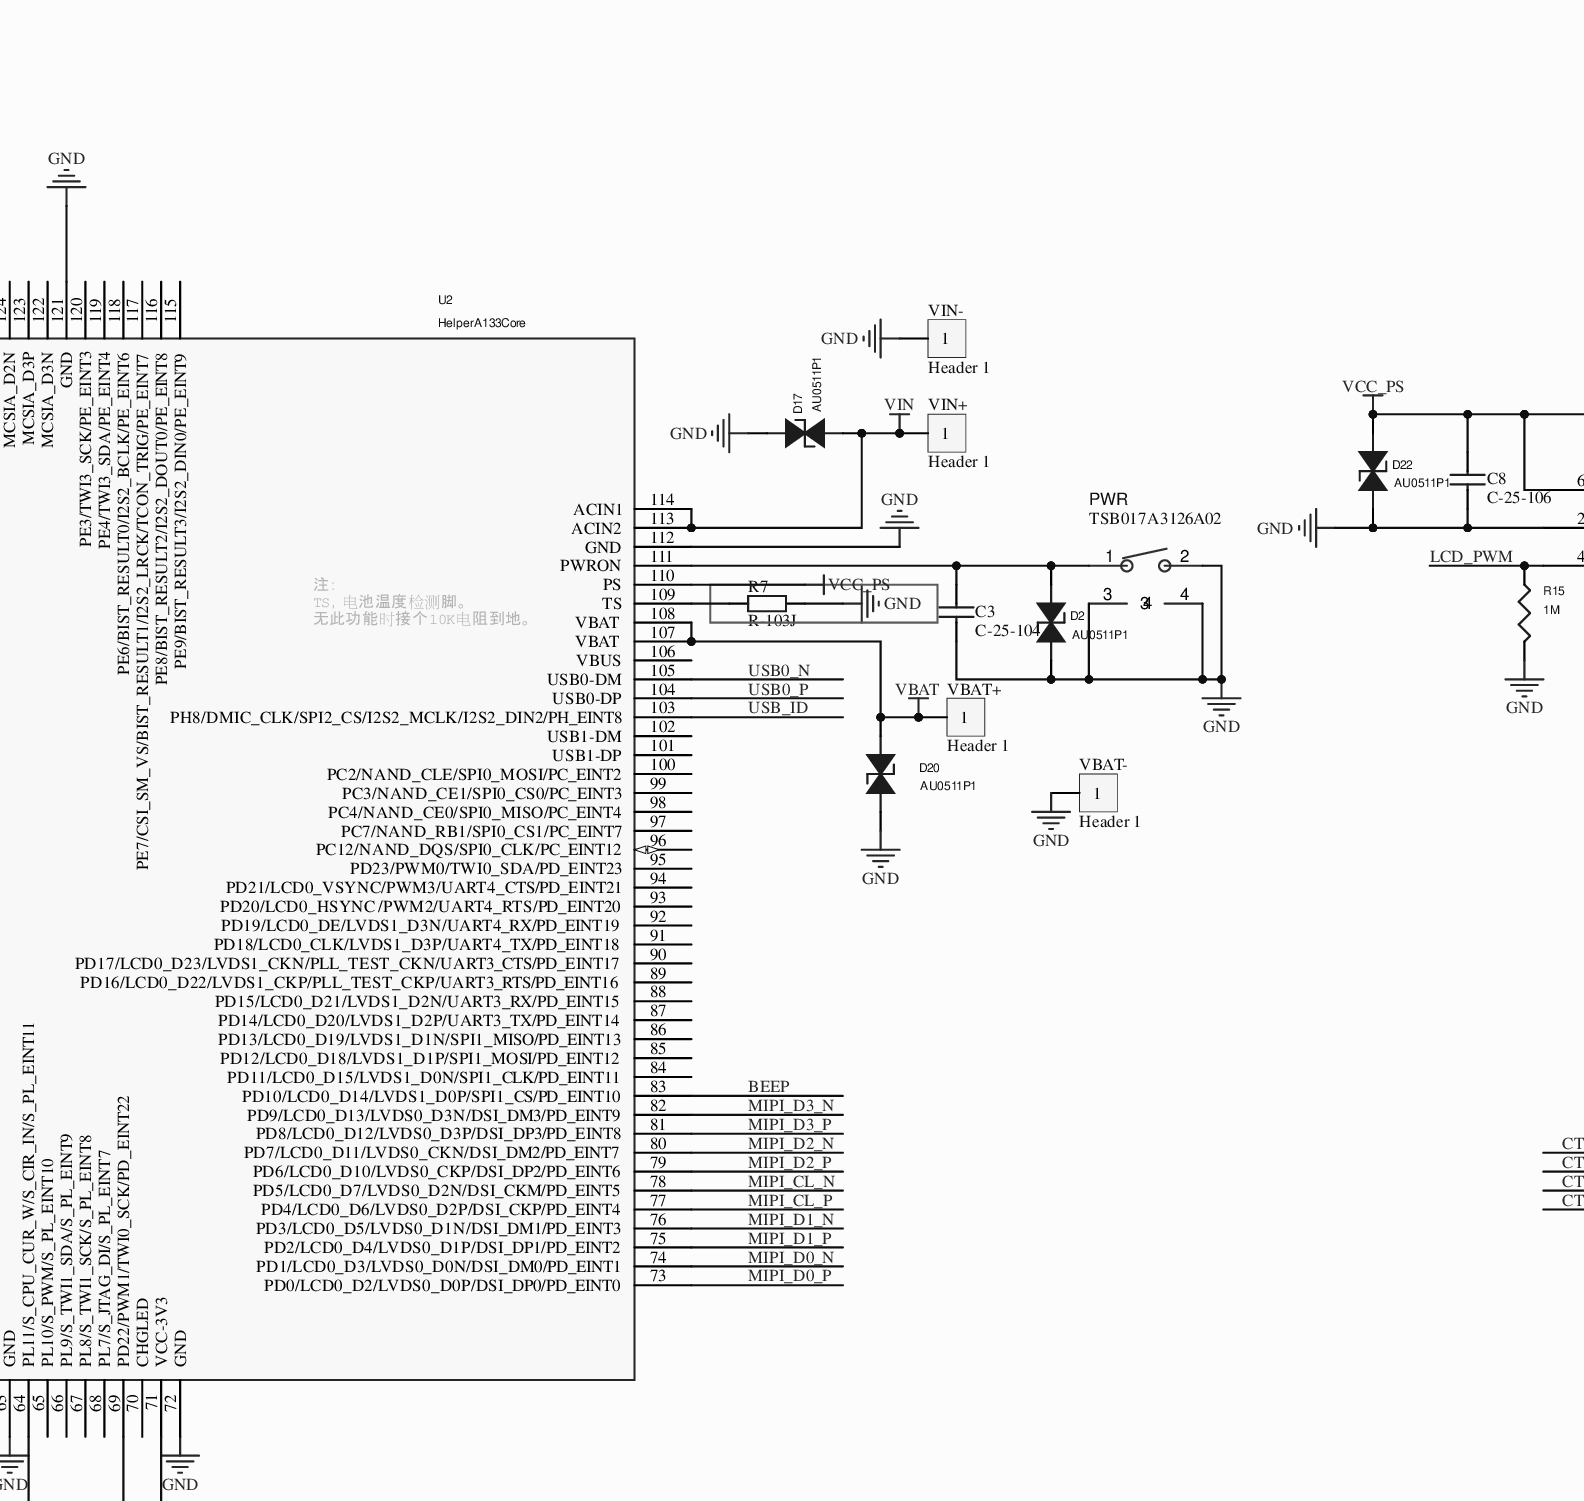
[diagram p0: MISC105407.SchDoc, centre column 3 of 4]
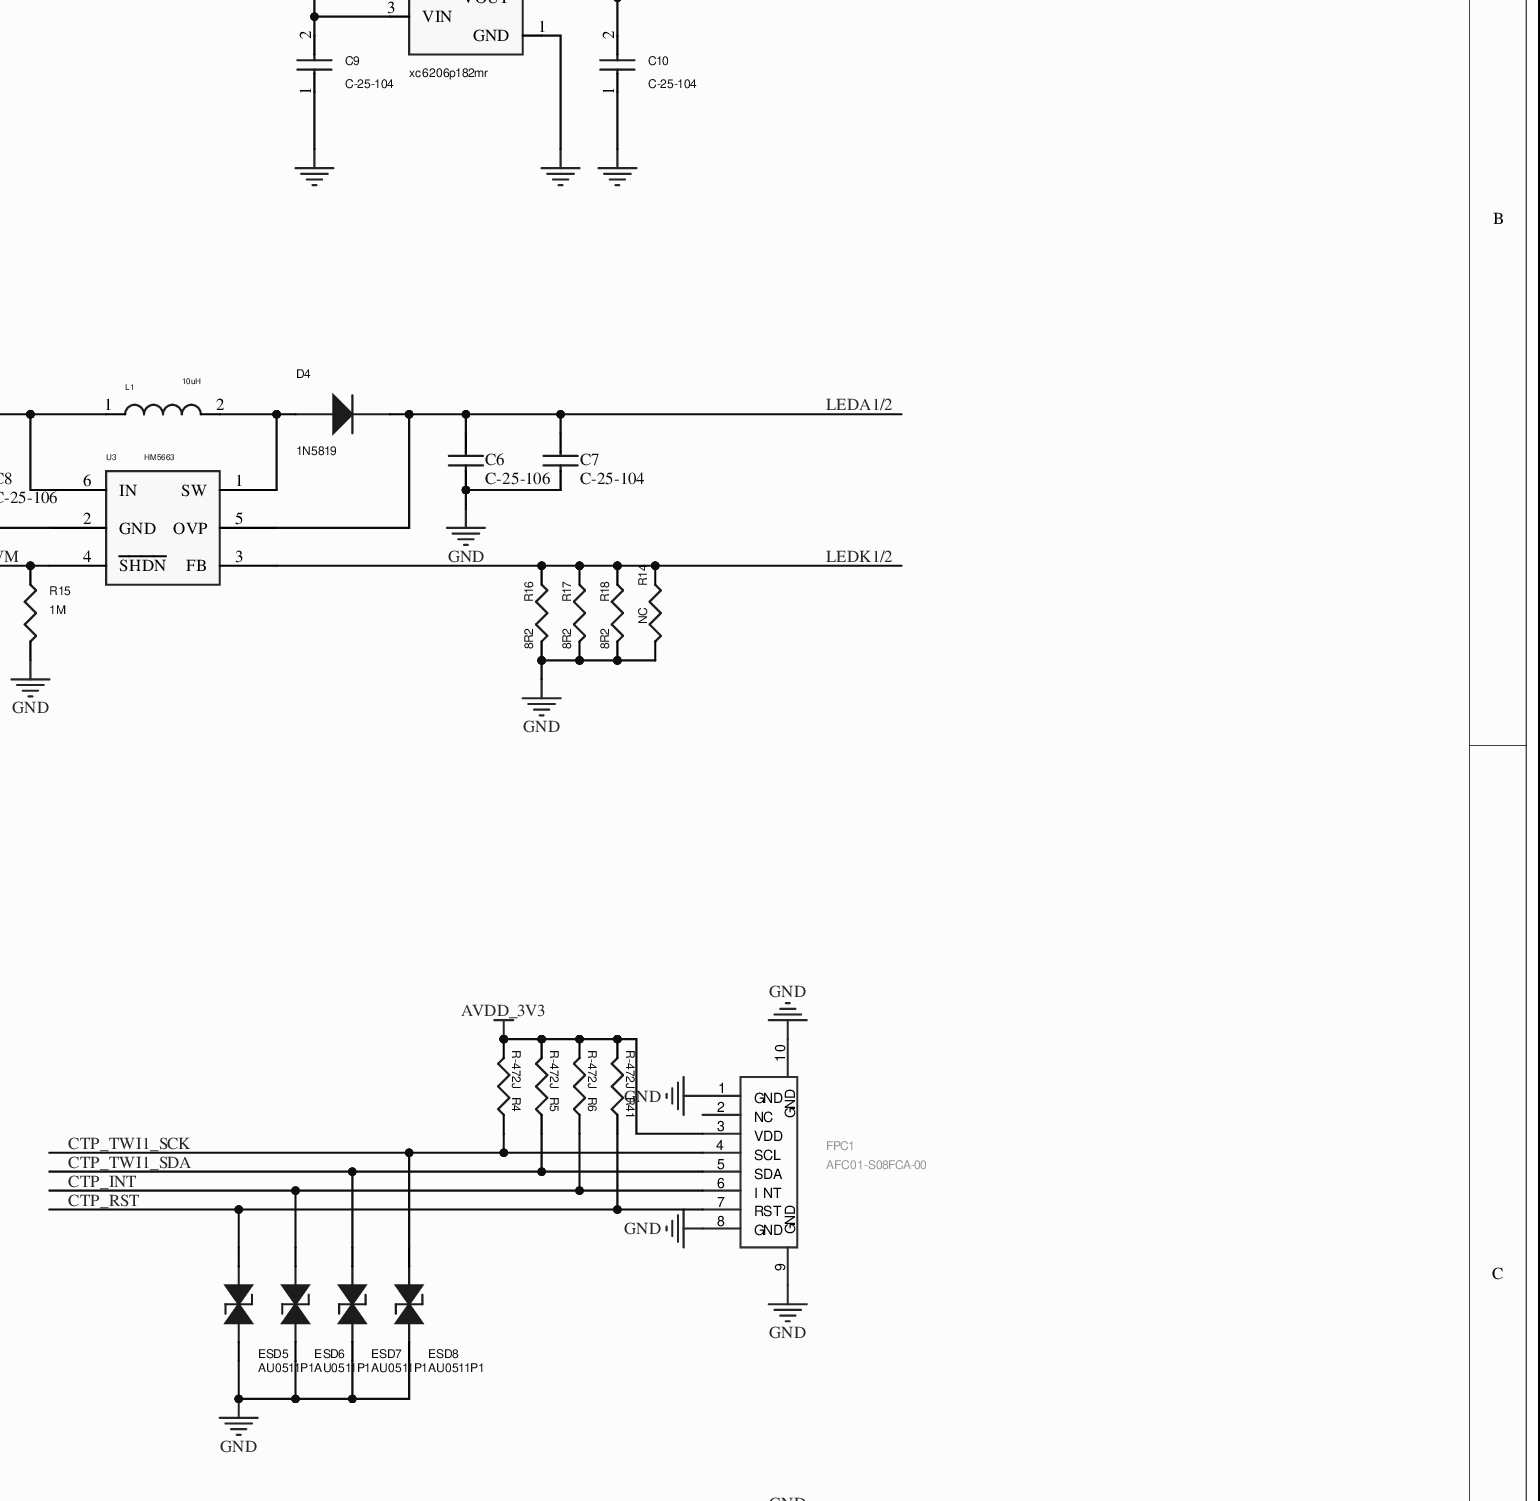
[diagram p1: MISC105407.SchDoc, centre column 4 of 4]
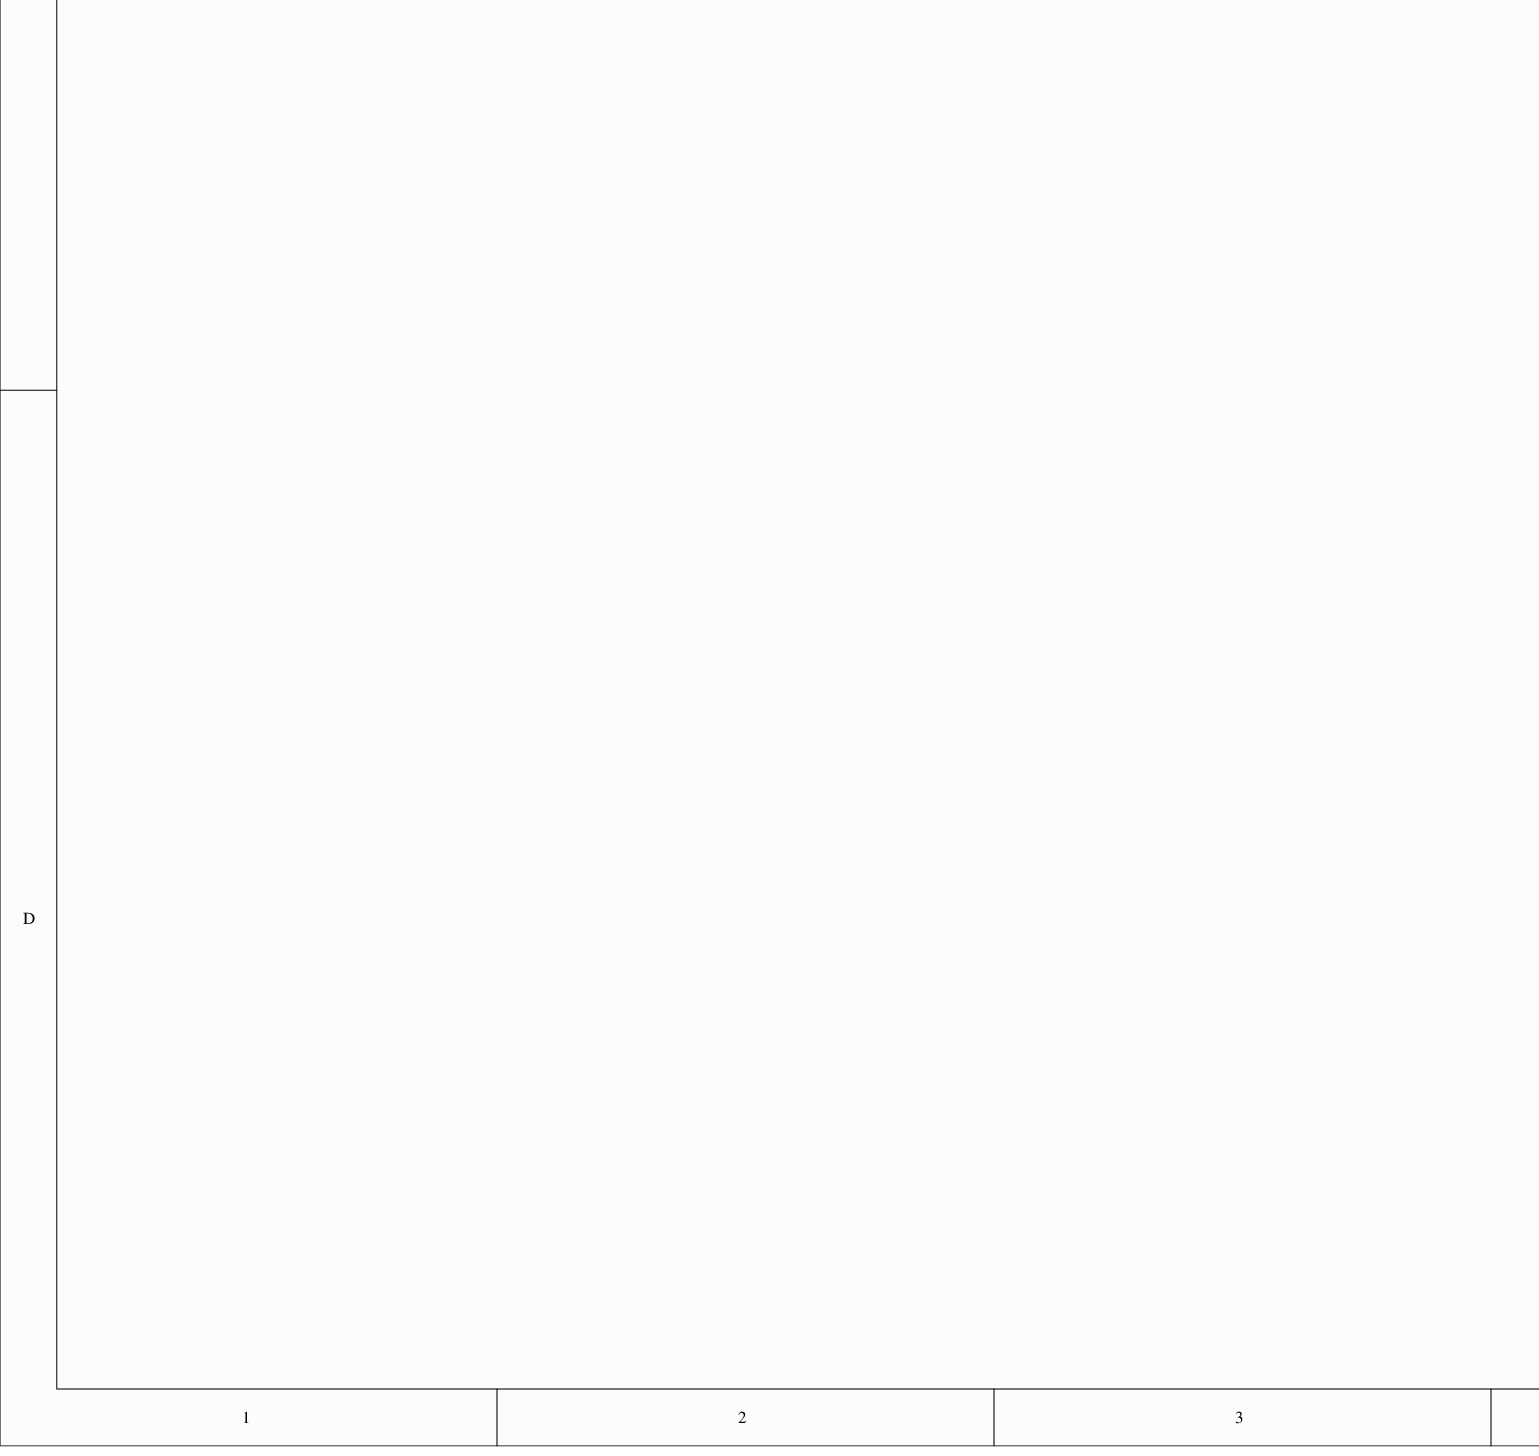
[diagram p2: MISC105407.SchDoc, bottom column 1 of 4]
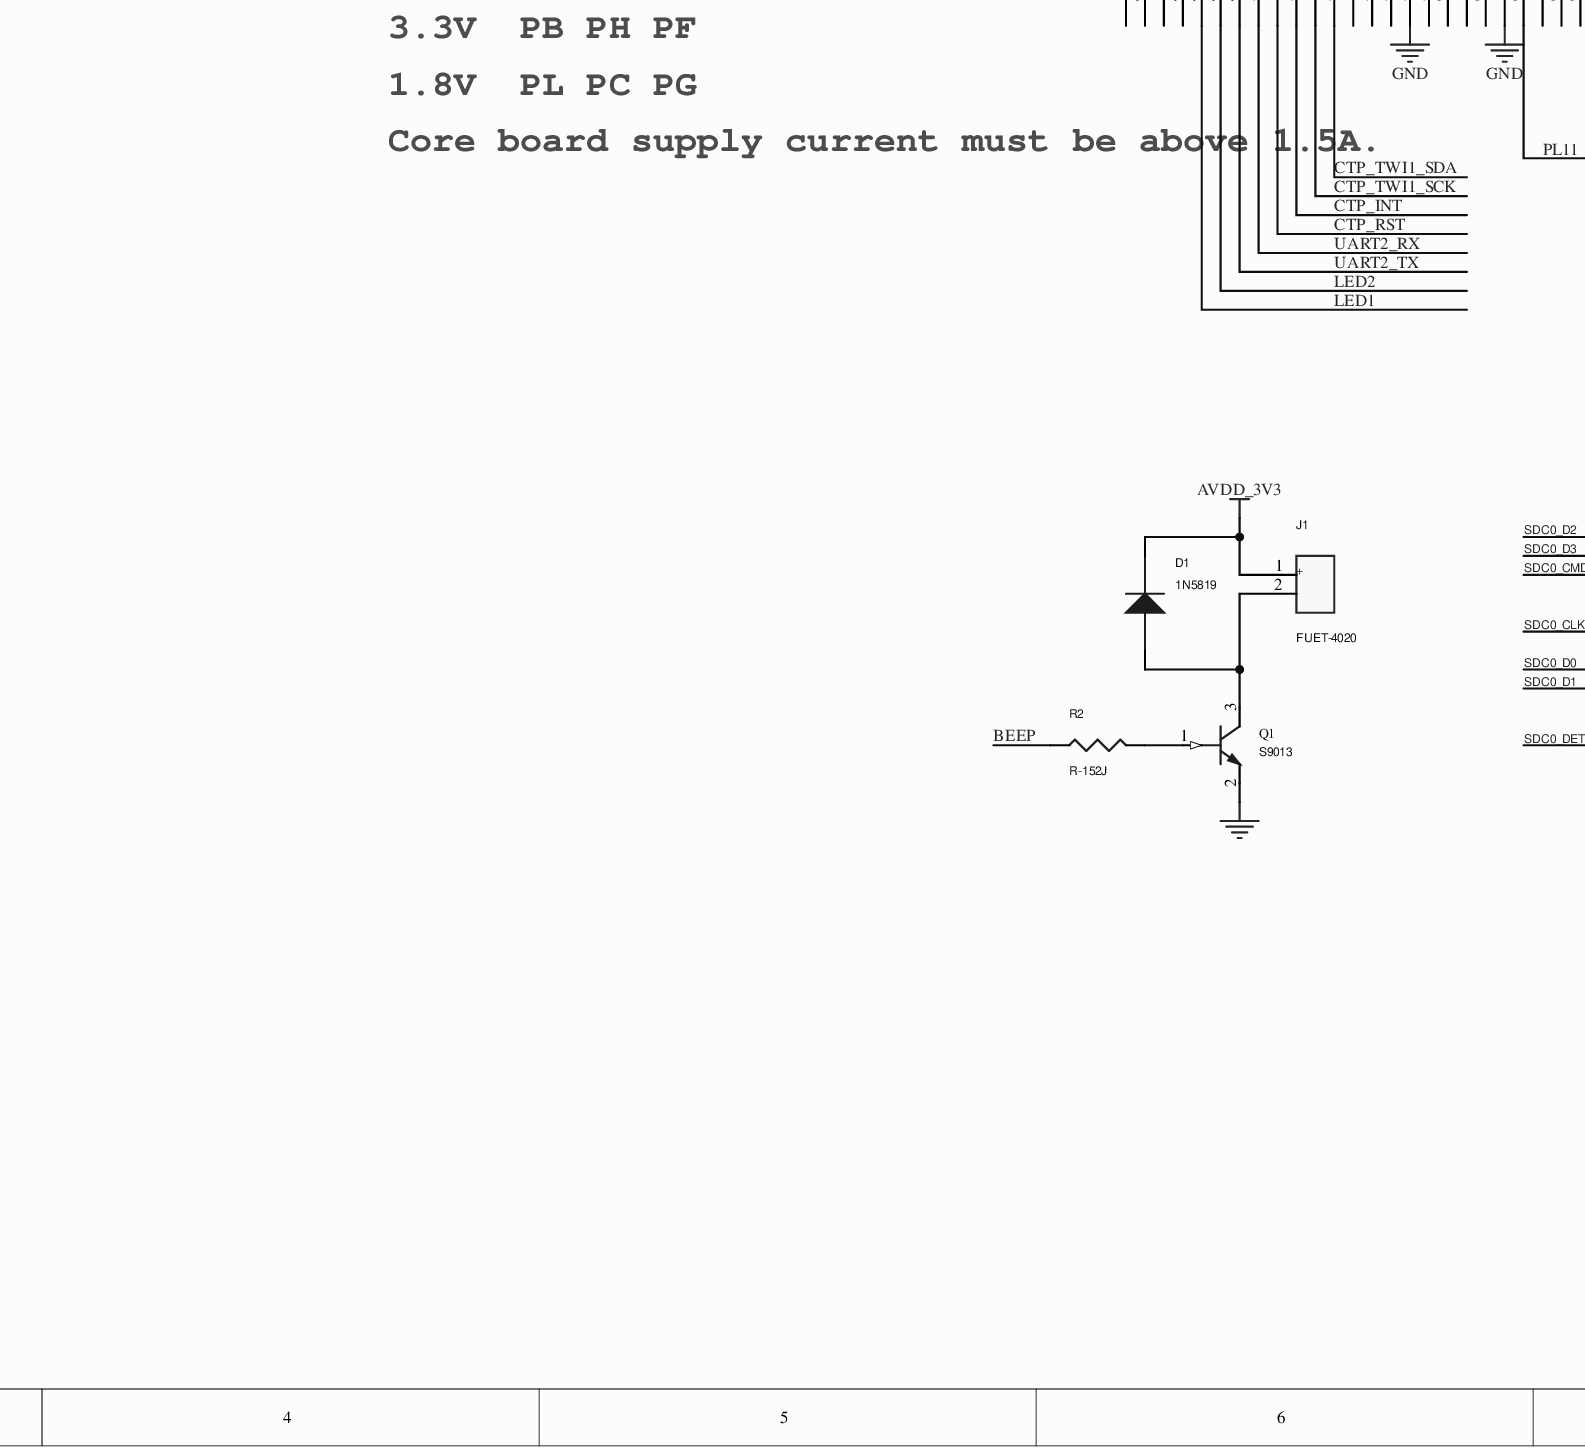
[diagram p3: MISC105407.SchDoc, bottom column 2 of 4]
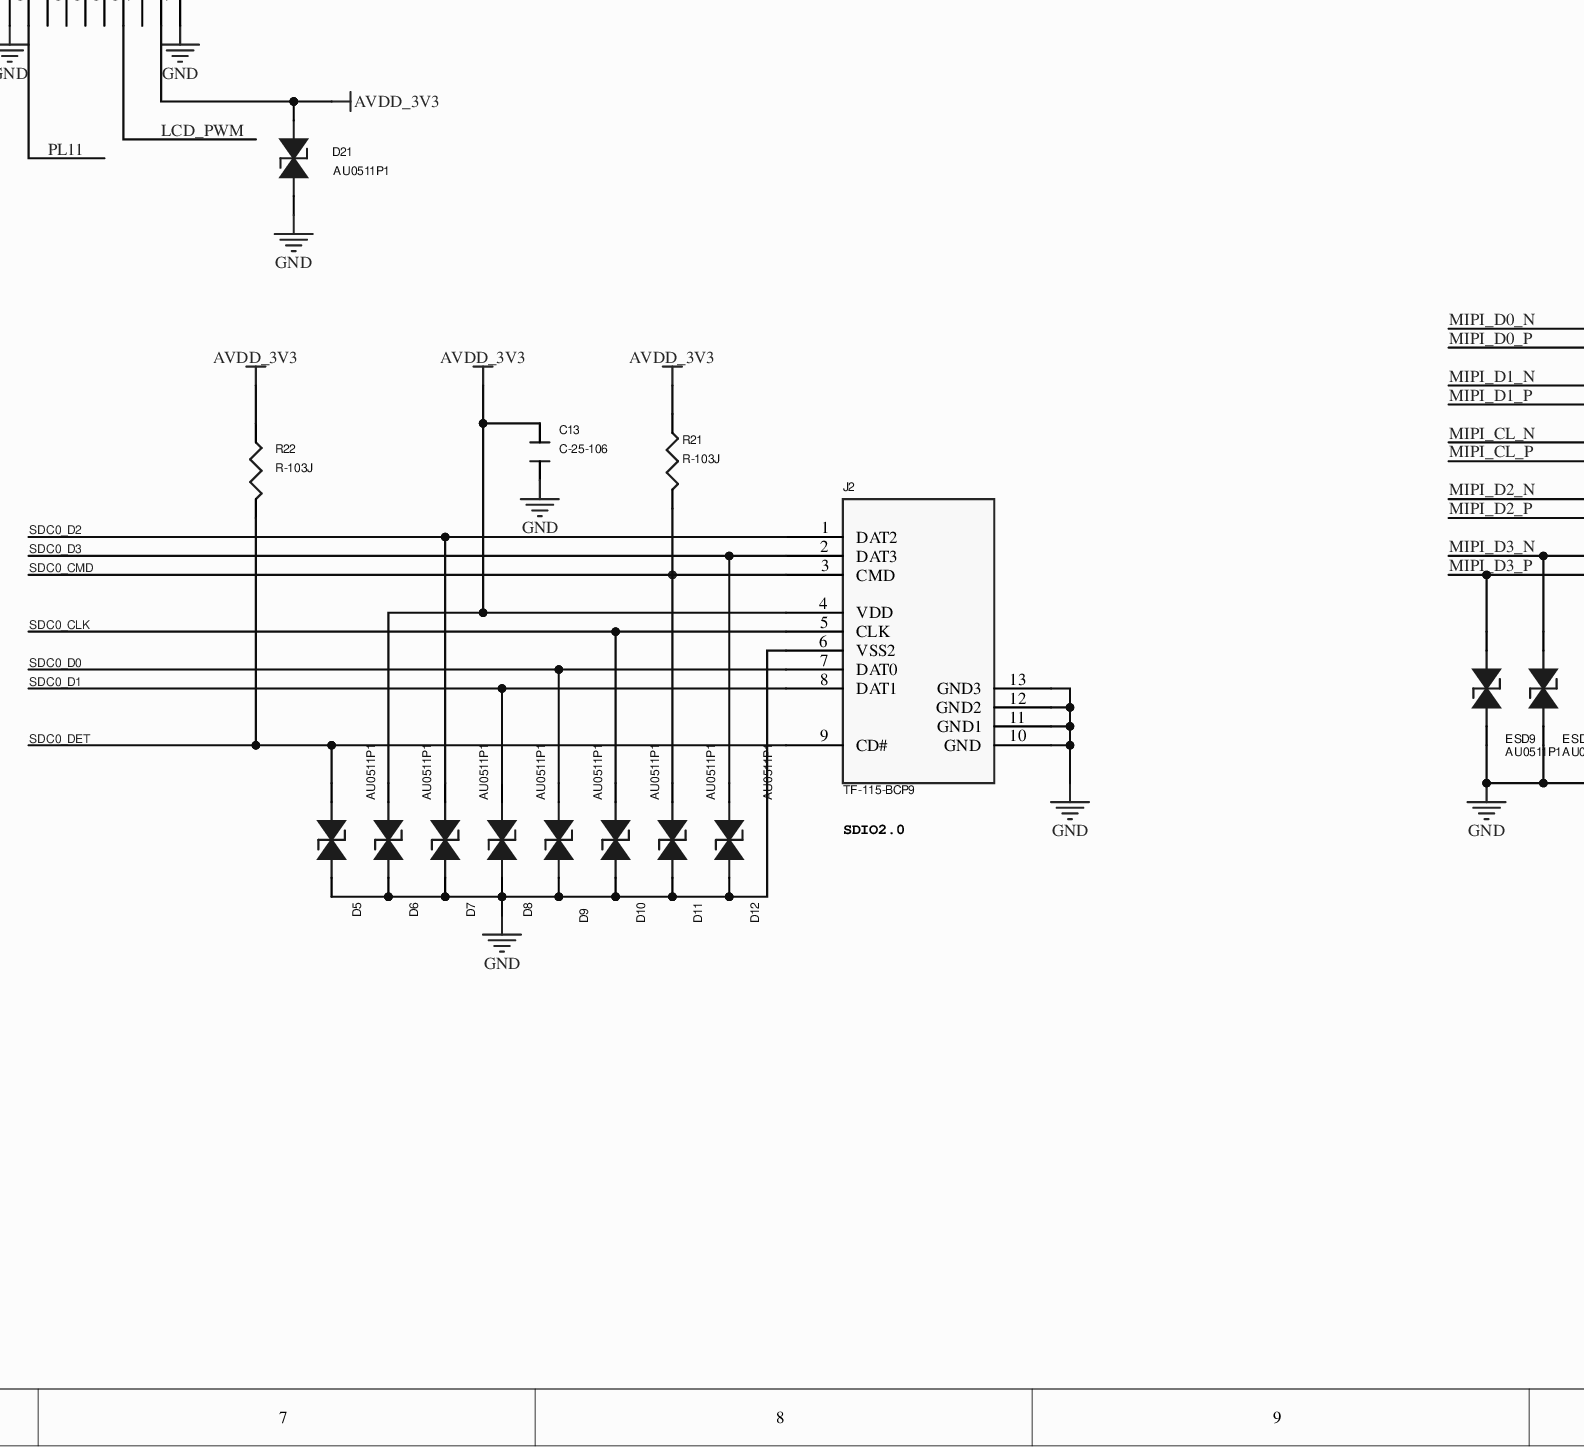
[diagram p4: MISC105407.SchDoc, bottom column 3 of 4]
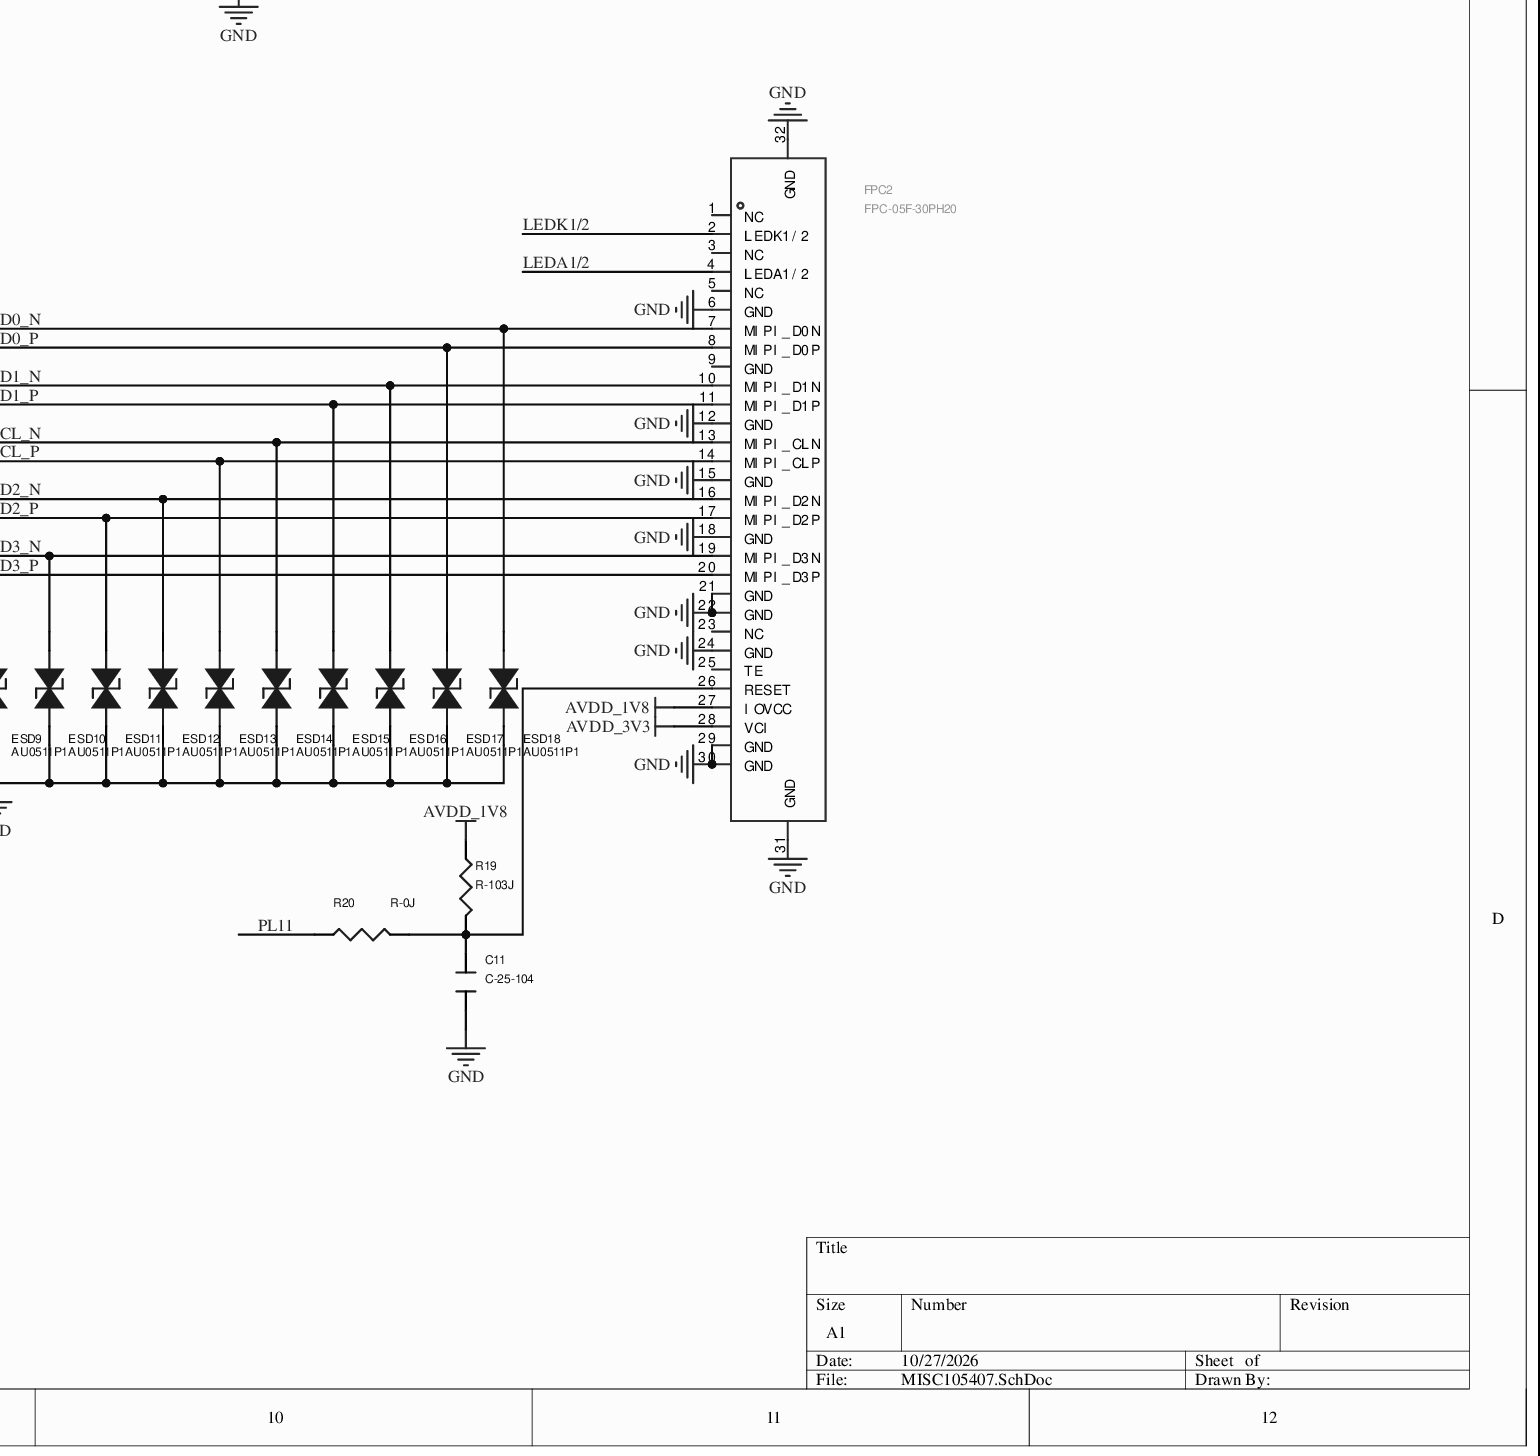
[diagram p5: MISC105407.SchDoc, bottom column 4 of 4]
# Altium project MISC105407.PrjPcb (part 2 of 3)
Board file: MISC105407.PcbDoc